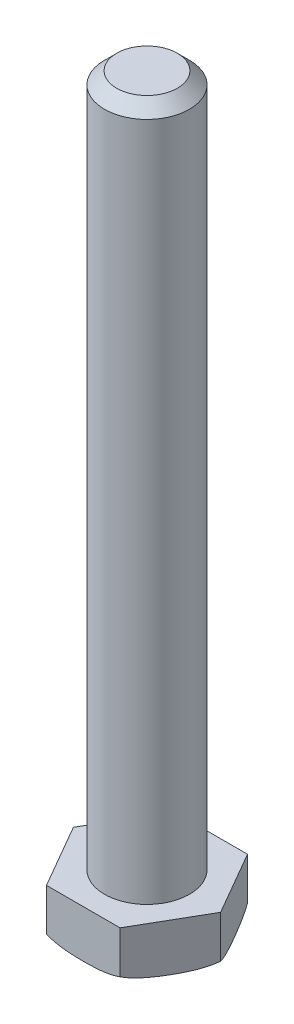
from build123d import *

# Parameters (mm, degrees)
BOSS_EXTRUDE1_DEPTH = 8
SKETCH2_R           = 7
BOSS_EXTRUDE2_DEPTH = 114
CHAMFER1_SIZE       = 2
SCALE_1_SCALE       = 1.875


with BuildPart() as part:
    # Sketch1 → Boss-Extrude1 (new body)
    with BuildSketch(Plane(origin=(0, 0, 0), x_dir=(1, 0, 0), z_dir=(0, 1, 0))):
        Polygon((12.124355653, 0), (6.062177826, 10.5), (-6.062177826, 10.5), (-12.124355653, 0), (-6.062177826, -10.5), (6.062177826, -10.5), align=None)
    extrude(amount=BOSS_EXTRUDE1_DEPTH)

    # Sketch2 → Boss-Extrude2 (add)
    with BuildSketch(Plane(origin=(0, 8, 0), x_dir=(1, 0, 0), z_dir=(0, 1, 0))):
        with Locations(Location((0, 0, 0), (0, 0, 90))):
            Circle(SKETCH2_R)
    extrude(amount=BOSS_EXTRUDE2_DEPTH)

    # Chamfer1
    chamfer1_edges = [part.edges().sort_by_distance(p)[0] for p in [
        (0, 122, 7),
    ]]
    chamfer(chamfer1_edges, length=CHAMFER1_SIZE)

    # Sketch3 → Cut-Revolve1 (revolve, cut)
    with BuildSketch(Plane.XY, mode=Mode.PRIVATE) as cut_revolve1_sk:
        with BuildLine():
            Line((-12.124355653, 0), (-12.124355653, 1))
            ThreePointArc((-12.124355653, 1), (-10.705494483, 0.25658351), (-9.124355653, 0))
            Line((-9.124355653, 0), (-12.124355653, 0))
        make_face()
    revolve(cut_revolve1_sk.sketch.rotate(Axis((0, 0, 0), (0, 1, 0)), 270), axis=Axis((0, 0, 0), (0, 1, 0)), mode=Mode.SUBTRACT)


with BuildPart() as part_1:
    # Scale 1: scaled about (-1.43e-07, 55.752743575, -2.4e-08)
    add(part.part.scale(SCALE_1_SCALE).moved(Location((1.25e-07, -48.783650628, 2.1e-08))))


solid = part_1.part
